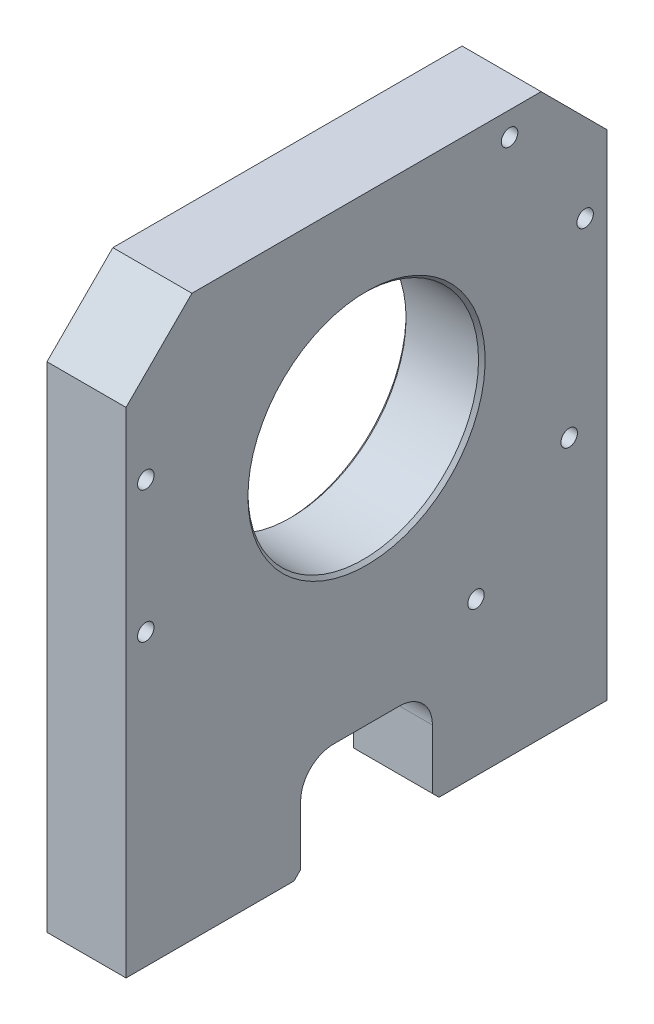
from build123d import *

# Parameters (mm, degrees)
SKETCH1_R             = 17.5
BOSS_EXTRUDE1_DEPTH   = 6
CHAMFER1_SIZE         = 10
M6_TAPPED_HOLE1_D     = 5
M6_TAPPED_HOLE1_DEPTH = 17
M6_TAPPED_HOLE1_TIP   = 1.502151548
SKETCH8_R             = 2
CUT_EXTRUDE1_DEPTH    = 15
CHAMFER2_SIZE         = 1
M3_TAPPED_HOLE1_D     = 2.5
CHAMFER3_SIZE         = 0.5


with BuildPart() as part:
    # Sketch1 → Boss-Extrude1 (new, symmetric)
    with BuildSketch(Plane(origin=(0, 0, 0), x_dir=(0, 0, -1), z_dir=(1, 0, 0))):
        with BuildLine():
            Line((-36.5, 0), (-10, 0))
            Line((-10, 0), (-10, 10))
            ThreePointArc((-10, 10), (-8.535533906, 13.535533906), (-5, 15))
            Line((-5, 15), (5, 15))
            ThreePointArc((5, 15), (8.535533906, 13.535533906), (10, 10))
            Line((10, 10), (10, 0))
            Line((10, 0), (36.5, 0))
            Line((36.5, 0), (36.5, 85))
            Line((36.5, 85), (-36.5, 85))
            Line((-36.5, 85), (-36.5, 0))
        make_face()
        with Locations((0, 54)):
            Circle(SKETCH1_R, mode=Mode.SUBTRACT)
    extrude(amount=BOSS_EXTRUDE1_DEPTH, both=True)

    # Chamfer1
    chamfer1_edges = [part.edges().sort_by_distance(p)[0] for p in [
        (0, 85, 36.5),
        (0, 85, -36.5),
    ]]
    chamfer(chamfer1_edges, length=CHAMFER1_SIZE)

    # M6 Tapped Hole1
    with Locations(Plane(origin=(0, 0, 0), x_dir=(-1, 0, 0), z_dir=(0, -1, 0))):
        with Locations((0, -25), (0, 25)):
            Hole(M6_TAPPED_HOLE1_D / 2, depth=M6_TAPPED_HOLE1_DEPTH)
            with Locations((0, 0, -(M6_TAPPED_HOLE1_DEPTH + M6_TAPPED_HOLE1_TIP / 2))):  # 118° drill point
                Cone(0, M6_TAPPED_HOLE1_D / 2, M6_TAPPED_HOLE1_TIP, mode=Mode.SUBTRACT)

    # Sketch8 → Cut-Extrude1 (cut)
    with BuildSketch(Plane.XZ):
        with Locations(Location((0, -15, 0), (0, 0, 270))):
            Circle(SKETCH8_R)
        with BuildLine():
            Line((2, 15.5), (2, 14.5))
            ThreePointArc((2, 14.5), (0, 12.5), (-2, 14.5))
            Line((-2, 14.5), (-2, 15.5))
            ThreePointArc((-2, 15.5), (0, 17.5), (2, 15.5))
        make_face()
    extrude(amount=-CUT_EXTRUDE1_DEPTH, mode=Mode.SUBTRACT)

    # Chamfer2
    chamfer2_edges = [part.edges().sort_by_distance(p)[0] for p in [
        (0, 0, -10),
        (0, 0, 10),
    ]]
    chamfer(chamfer2_edges, length=CHAMFER2_SIZE)

    # M3 Tapped Hole1 (through all)
    with Locations(Plane.ZY.offset(6)):
        with Locations((33.5, 44), (33.5, 64), (-16.617009358, 23.240855018), (-30.759144982, 37.382990642), (-33.177357847, 65.023290175), (-21.70582912, 81.406331061)):
            Hole(M3_TAPPED_HOLE1_D / 2)

    # Chamfer3
    chamfer3_edges = [part.edges().sort_by_distance(p)[0] for p in [
        (-6, 54, 17.5),
        (6, 54, 17.5),
    ]]
    chamfer(chamfer3_edges, length=CHAMFER3_SIZE)


solid = part.part
